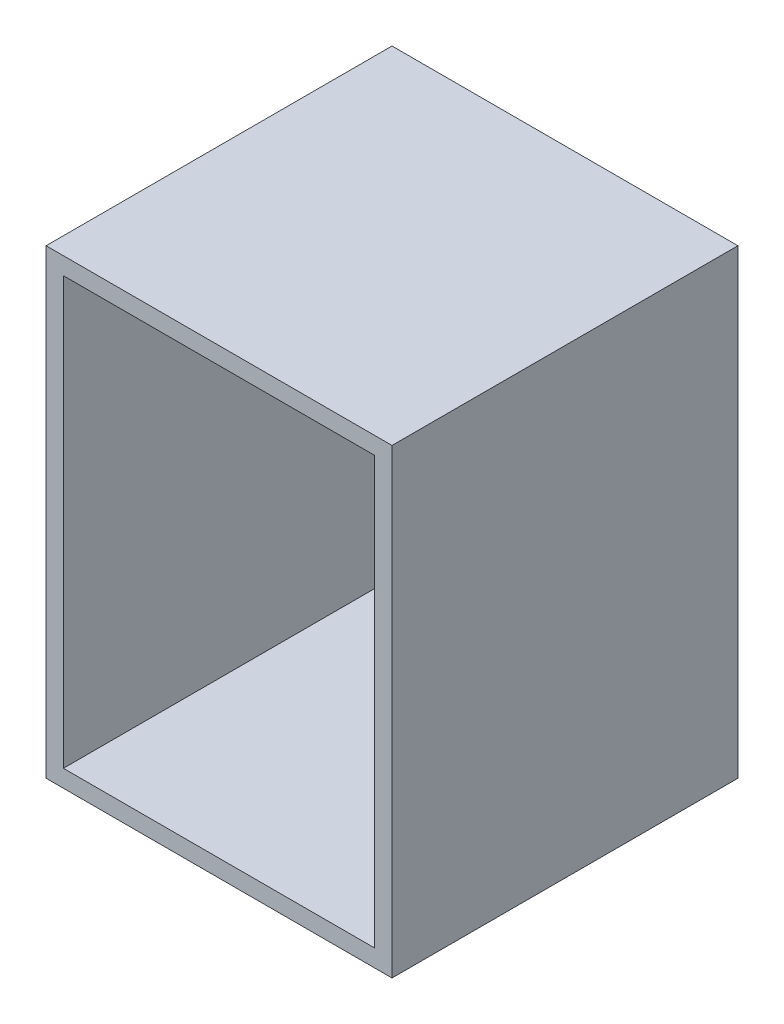
from build123d import *

# Parameters (mm, degrees)
SKETCH1_W           = 30
SKETCH1_H           = 40
BOSS_EXTRUDE1_DEPTH = 30
SKETCH2_W           = 27
SKETCH2_H           = 37
CUT_EXTRUDE1_DEPTH  = 62.755555196


with BuildPart() as part:
    # Sketch1 → Boss-Extrude1 (new body)
    with BuildSketch(Plane.XY):
        with Locations((-22.059069992, 19.247597747)):
            Rectangle(SKETCH1_W, SKETCH1_H)
    extrude(amount=BOSS_EXTRUDE1_DEPTH)

    # Sketch2 → Cut-Extrude1 (cut, through all)
    with BuildSketch(Plane.XY.offset(30)):
        with Locations((-22.059069992, 19.247597747)):
            Rectangle(SKETCH2_W, SKETCH2_H)
    extrude(amount=-CUT_EXTRUDE1_DEPTH, mode=Mode.SUBTRACT)


solid = part.part
